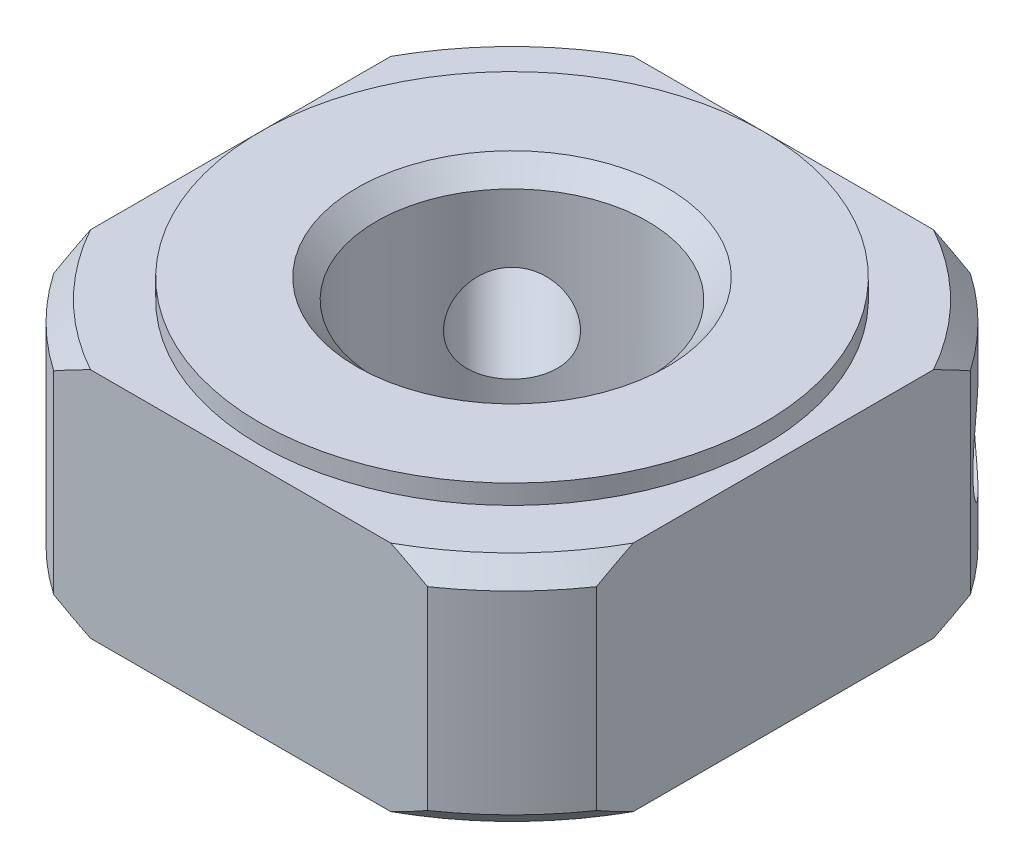
from build123d import *

# Parameters (mm, degrees)
SKETCH1_R                 = 6.5
BOSS_EXTRUDE1_DEPTH       = 0.5
SKETCH3_R                 = 8.5
BOSS_EXTRUDE3_DEPTH       = 6
CHAMFER2_SIZE             = 0.5
SKETCH4_W                 = 4.01520781
SKETCH4_H                 = 18.659876277
SKETCH4_W_2               = 10.097066699
SKETCH4_H_2               = 2.598075642
SKETCH4_W_3               = 5.358269855
SKETCH4_H_3               = 23.485379118
SKETCH4_W_4               = 10.284722044
SKETCH4_H_4               = 2.952358684
CUT_EXTRUDE3_DEPTH        = 14.435028843
M8X1_0_TAPPED_HOLE1_D     = 7
M8X1_0_TAPPED_HOLE1_DEPTH = 19
M8X1_0_TAPPED_HOLE1_TIP   = 2.103012167
SKETCH7_W                 = 1.25
SKETCH7_H                 = 9.899494937
CHAMFER3_SIZE             = 0.5
CIRPATTERN1_COUNT         = 2
CIRPATTERN1_ANGLE         = 90


with BuildPart() as part:
    # Sketch1 → Boss-Extrude1 (new body)
    with BuildSketch(Plane(origin=(0, 0, 0), x_dir=(1, 0, 0), z_dir=(0, 1, 0))):
        with Locations(Location((0, 0, 0), (0, 0, 270))):
            Circle(SKETCH1_R)
    extrude(amount=BOSS_EXTRUDE1_DEPTH)

    # Sketch3 → Boss-Extrude3 (add)
    with BuildSketch(Plane.XZ):
        with Locations(Location((0, 0, 0), (0, 0, 270))):
            Circle(SKETCH3_R)
    extrude(amount=BOSS_EXTRUDE3_DEPTH)

    # Chamfer2
    chamfer2_edges = [part.edges().sort_by_distance(p)[0] for p in [
        (0, 0, 8.5),
        (0, -6, 8.5),
    ]]
    chamfer(chamfer2_edges, length=CHAMFER2_SIZE)

    # Sketch4 → Cut-Extrude3 (cut, through all)
    with BuildSketch(Plane(origin=(0, 0, 0), x_dir=(1, 0, 0), z_dir=(0, 1, 0))):
        with Locations((-9.007603905, 1.516224116)):
            Rectangle(SKETCH4_W, SKETCH4_H)
        with Locations((0.059047173, 8.299037821)):
            Rectangle(SKETCH4_W_2, SKETCH4_H_2)
        with Locations((9.679134928, -0.60539293)):
            Rectangle(SKETCH4_W_3, SKETCH4_H_3)
        with Locations((-0.142361022, -8.476179342)):
            Rectangle(SKETCH4_W_4, SKETCH4_H_4)
    extrude(amount=-CUT_EXTRUDE3_DEPTH, mode=Mode.SUBTRACT)

    # M8x1.0 Tapped Hole1
    with Locations(Plane(origin=(0, 0.5, 0), x_dir=(-1, 0, 0), z_dir=(0, 1, 0))):
        with Locations((0, 0)):
            Hole(M8X1_0_TAPPED_HOLE1_D / 2, depth=M8X1_0_TAPPED_HOLE1_DEPTH)
            with Locations((0, 0, -(M8X1_0_TAPPED_HOLE1_DEPTH + M8X1_0_TAPPED_HOLE1_TIP / 2))):  # 118° drill point
                Cone(0, M8X1_0_TAPPED_HOLE1_D / 2, M8X1_0_TAPPED_HOLE1_TIP, mode=Mode.SUBTRACT)

    # Sketch7 → M3 Tapped Hole1 (revolve, cut)
    with BuildSketch(Plane(origin=(0, -3, 0), x_dir=(0.7071067811865488, 0, 0.7071067811865464), z_dir=(0, 1, 0))):
        with Locations((0.625, 4.949747469)):
            Rectangle(SKETCH7_W, SKETCH7_H)
    m3_tapped_hole1 = revolve(axis=Axis((-4.490128061, -3, 4.490128061), (0.7071067811865464, 0, -0.7071067811865487)), mode=Mode.SUBTRACT)

    # Chamfer3
    chamfer3_edges = [part.edges().sort_by_distance(p)[0] for p in [
        (-3.5, -6, 0),
        (-3.5, 0.5, 0),
    ]]
    chamfer(chamfer3_edges, length=CHAMFER3_SIZE)

    # CirPattern1: M3 Tapped Hole1 ×2 about axis
    cirpattern1_axis = Axis((0, 0.5, 0), (0, 1, 0))
    for i in range(1, CIRPATTERN1_COUNT):
        add(m3_tapped_hole1.rotate(cirpattern1_axis, i * CIRPATTERN1_ANGLE / (CIRPATTERN1_COUNT - 1)), mode=Mode.SUBTRACT)


solid = part.part
